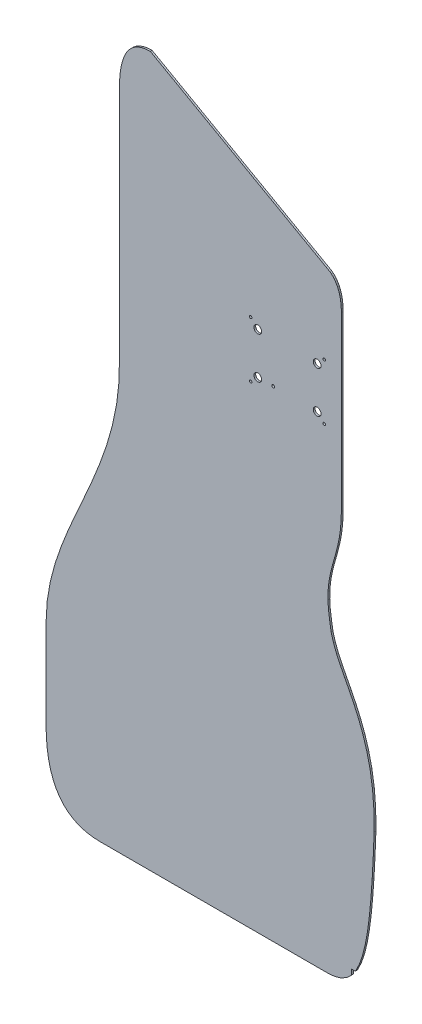
from build123d import *

# Parameters (mm, degrees)
EXTRUDE_1_DEPTH     = 1.5
SKETCH_2_W          = 32
SKETCH_2_H          = 22
CUT_EXTRUDE_1_DEPTH = 10
SKETCH_3_R          = 2.25
SKETCH_3_R_2        = 6.5
CUT_EXTRUDE_2_DEPTH = 5


with BuildPart() as part:
    # 草图1 → 凸台-拉伸1 (new, symmetric)
    with BuildSketch(Plane.XY):
        Polygon((103, 235), (-24.833333333, 235), (-152.666666667, 235), (-280.5, 235), (-293.035714286, 235.637755102), (-304.642857143, 237.551020408), (-315.321428571, 240.739795918), (-325.071428571, 245.204081633), (-333.892857143, 250.943877551), (-341.785714286, 257.959183673), (-348.75, 266.25), (-354.785714286, 275.816326531), (-359.892857143, 286.658163265), (-364.071428571, 298.775510204), (-367.321428571, 312.168367347), (-369.642857143, 326.836734694), (-371.035714286, 342.780612245), (-371.5, 360), (-371.5, 410), (-371.5, 460), (-371.5, 510), (-369.607325073, 541.716472303), (-364.317784257, 572.711370262), (-356.214103499, 603.18148688), (-345.879008746, 633.32361516), (-333.895225948, 663.334548105), (-320.84548105, 693.411078717), (-307.3125, 723.75), (-293.879008746, 754.548104956), (-281.127733236, 786.002186589), (-269.641399417, 818.309037901), (-260.002733236, 851.665451895), (-252.794460641, 886.268221574), (-248.59930758, 922.314139942), (-248, 960), (-248, 1090), (-248, 1220), (-248, 1350), (-247.734693878, 1361.020408163), (-246.93877551, 1371.224489796), (-245.612244898, 1380.612244898), (-243.755102041, 1389.183673469), (-241.367346939, 1396.93877551), (-238.448979592, 1403.87755102), (-235, 1410), (-231.020408163, 1415.306122449), (-226.510204082, 1419.795918367), (-221.469387755, 1423.469387755), (-215.897959184, 1426.326530612), (-209.795918367, 1428.367346939), (-203.163265306, 1429.591836735), (-196, 1430), (-95.25, 1373.333333333), (5.5, 1316.666666667), (106.25, 1260), (108.93622449, 1257.887755102), (111.423469388, 1255.551020408), (113.711734694, 1252.989795918), (115.801020408, 1250.204081633), (117.691326531, 1247.193877551), (119.382653061, 1243.959183673), (120.875, 1240.5), (122.168367347, 1236.816326531), (123.262755102, 1232.908163265), (124.158163265, 1228.775510204), (124.854591837, 1224.418367347), (125.352040816, 1219.836734694), (125.650510204, 1215.030612245), (125.75, 1210), (125.75, 1113.333333333), (125.75, 1016.666666667), (125.75, 920), (125.280976676, 904.7303207), (123.987609329, 890.903790087), (122.040451895, 878.279883382), (119.610058309, 866.618075802), (116.866982507, 855.677842566), (113.981778426, 845.218658892), (111.125, 835), (108.467201166, 824.781341108), (106.17893586, 814.322157434), (104.430758017, 803.381924198), (103.393221574, 791.720116618), (103.236880466, 779.096209913), (104.13228863, 765.2696793), (106.25, 750), (108.586825802, 735.40451895), (112.60787172, 721.39941691), (118.007561953, 707.656705539), (124.4803207, 693.848396501), (131.720572157, 679.646501458), (139.422740525, 664.72303207), (147.28125, 648.75), (154.990524781, 631.39941691), (162.244989067, 612.343294461), (168.739067055, 591.253644315), (174.167182945, 567.802478134), (178.223760933, 541.66180758), (180.603225219, 512.503644315), (181, 480), (179.493440233, 443.170553936), (177.702623907, 409.752186589), (175.542274052, 379.635568513), (172.927113703, 352.711370262), (169.771865889, 328.870262391), (165.991253644, 308.002915452), (161.5, 290), (156.212827988, 274.752186589), (150.044460641, 262.150145773), (142.909620991, 252.084548105), (134.72303207, 244.44606414), (125.39941691, 239.125364431), (114.853498542, 236.013119534), align=None)
    extrude(amount=EXTRUDE_1_DEPTH, both=True)

    # 草图2 → 切除-拉伸1 (cut, symmetric)
    with BuildSketch(Plane.XY):
        with Locations((159, 250)):
            Rectangle(SKETCH_2_W, SKETCH_2_H)
        with Locations((159, 1150)):
            Rectangle(SKETCH_2_W, SKETCH_2_H)
    extrude(amount=CUT_EXTRUDE_1_DEPTH, both=True, mode=Mode.SUBTRACT)

    # 草图3 → 切除-拉伸2 (cut, symmetric)
    with BuildSketch(Plane.XY):
        with Locations(Location((-27, 1127, 0), (0, 0, 180))):
            Circle(SKETCH_3_R)
        with Locations(Location((-27, 1033, 0), (0, 0, 180))):
            Circle(SKETCH_3_R)
        with Locations(Location((97, 1127, 0), (0, 0, 180))):
            Circle(SKETCH_3_R)
        with Locations(Location((97, 1033, 0), (0, 0, 180))):
            Circle(SKETCH_3_R)
        with Locations(Location((-15, 1115, 0), (0, 0, 180))):
            Circle(SKETCH_3_R_2)
        with Locations(Location((-15, 1045, 0), (0, 0, 180))):
            Circle(SKETCH_3_R_2)
        with Locations(Location((85, 1115, 0), (0, 0, 180))):
            Circle(SKETCH_3_R_2)
        with Locations(Location((85, 1045, 0), (0, 0, 180))):
            Circle(SKETCH_3_R_2)
        with Locations(Location((11, 1045, 0), (0, 0, 180))):
            Circle(SKETCH_3_R)
    extrude(amount=CUT_EXTRUDE_2_DEPTH, both=True, mode=Mode.SUBTRACT)


solid = part.part
